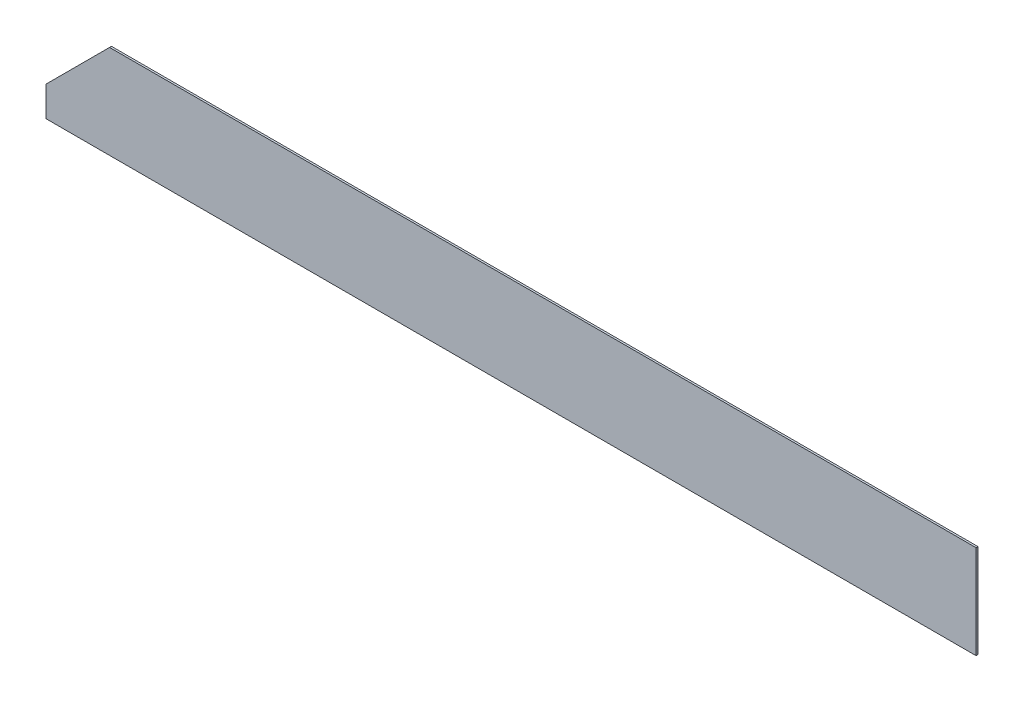
from build123d import *

# Parameters (mm, degrees)
BOSS_EXTRUDE1_DEPTH = 8


with BuildPart() as part:
    # Sketch1 → Boss-Extrude1 (new, symmetric)
    with BuildSketch(Plane.XY):
        Polygon((0, 0), (0, 780), (-7226, 780), (-7756, 250), (-7756, 0), align=None)
    extrude(amount=BOSS_EXTRUDE1_DEPTH, both=True)


solid = part.part
